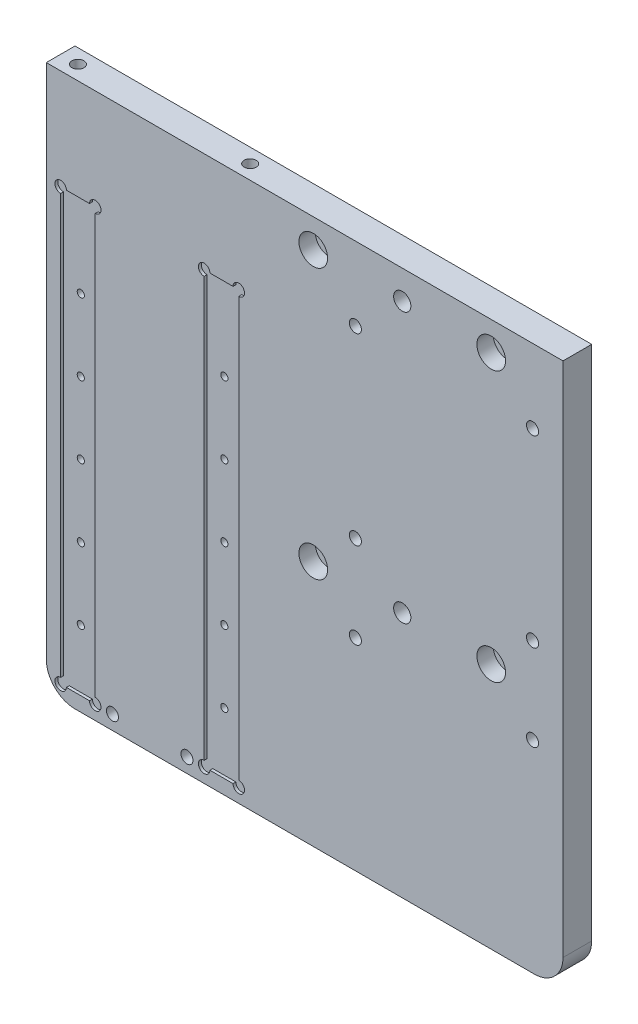
from build123d import *

# Parameters (mm, degrees)
SKETCH_1_W                = 180
SKETCH_1_H                = 190
EXTRUDE_1_DEPTH           = 10
HOLE_WIZARD_1_D           = 5.5
HOLE_WIZARD_1_CBORE_D     = 10
HOLE_WIZARD_1_CBORE_DEPTH = 5.7
PATTERN_LINEAR_1_COUNT    = 2
PATTERN_LINEAR_1_PITCH    = 94
SKETCH_4_W                = 12.05
SKETCH_4_H                = 150
CUT_EXTRUDE_1_DEPTH       = 1
SKETCH_6_R                = 2
CUT_EXTRUDE_2_DEPTH       = 1
HOLE_WIZARD_M5_1_D        = 4.2
HOLE_WIZARD_M5_1_DEPTH    = 14
HOLE_WIZARD_M5_1_TIP      = 1.2618073
FILLET_1_R                = 10
HOLE_WIZARD_M5_2_D        = 4.2
HOLE_WIZARD_M5_3_D        = 4.2
HOLE_WIZARD_6_0_6_1_D     = 6
HOLE_WIZARD_6_0_6_1_DEPTH = 10
HOLE_WIZARD_6_0_6_1_TIP   = 1.802581857
HOLE_WIZARD_M3_1_D        = 2.5


with BuildPart() as part:
    # 草图1 → 凸台-拉伸1 (new body)
    with BuildSketch(Plane.XY):
        with Locations((0, -95)):
            Rectangle(SKETCH_1_W, SKETCH_1_H)
    extrude(amount=EXTRUDE_1_DEPTH)

    # 打孔尺寸(%根据)开槽圆柱头螺钉的类型1 (through all)
    with Locations(Plane.XY.offset(10)):
        with Locations((65, -10), (3, -10)):
            hole_wizard_1 = CounterBoreHole(HOLE_WIZARD_1_D / 2, HOLE_WIZARD_1_CBORE_D / 2, HOLE_WIZARD_1_CBORE_DEPTH)

    # 阵列(线性)1: 打孔尺寸(%根据)开槽圆柱头螺钉的类型1 ×2
    with Locations(*[(0, -i * PATTERN_LINEAR_1_PITCH, 0) for i in range(1, PATTERN_LINEAR_1_COUNT)]):
        add(hole_wizard_1, mode=Mode.SUBTRACT)

    # 草图4 → 切除-拉伸1 (cut)
    with BuildSketch(Plane.XY.offset(10)):
        with Locations((-78.975, -110)):
            Rectangle(SKETCH_4_W, SKETCH_4_H)
        with Locations((-28.975, -110)):
            Rectangle(SKETCH_4_W, SKETCH_4_H)
    extrude(amount=-CUT_EXTRUDE_1_DEPTH, mode=Mode.SUBTRACT)

    # 草图6 → 切除-拉伸2 (cut)
    with BuildSketch(Plane.XY.offset(10)):
        with Locations((-72.95, -35)):
            Circle(SKETCH_6_R)
        with Locations((-85, -35)):
            Circle(SKETCH_6_R)
        with Locations((-85, -185)):
            Circle(SKETCH_6_R)
        with Locations((-72.95, -185)):
            Circle(SKETCH_6_R)
        with Locations((-35, -185)):
            Circle(SKETCH_6_R)
        with Locations((-22.95, -185)):
            Circle(SKETCH_6_R)
        with Locations((-35, -35)):
            Circle(SKETCH_6_R)
        with Locations((-22.95, -35)):
            Circle(SKETCH_6_R)
    extrude(amount=-CUT_EXTRUDE_2_DEPTH, mode=Mode.SUBTRACT)

    # M5 螺纹孔1
    with Locations(Plane(origin=(0, 0, 0), x_dir=(1, 0, 0), z_dir=(0, 1, 0))):
        with Locations((-23.975, -5), (-83.975, -5)):
            Hole(HOLE_WIZARD_M5_1_D / 2, depth=HOLE_WIZARD_M5_1_DEPTH)
            with Locations((0, 0, -(HOLE_WIZARD_M5_1_DEPTH + HOLE_WIZARD_M5_1_TIP / 2))):  # 118° drill point
                Cone(0, HOLE_WIZARD_M5_1_D / 2, HOLE_WIZARD_M5_1_TIP, mode=Mode.SUBTRACT)

    # 圆角1
    fillet_1_edges = [part.edges().sort_by_distance(p)[0] for p in [
        (90, -190, 5),
        (-90, -190, 5),
    ]]
    fillet(fillet_1_edges, radius=FILLET_1_R)

    # M5 螺纹孔2 (through all)
    with Locations(Plane.XY.offset(10)):
        with Locations((-66.95, -185), (-41, -185)):
            Hole(HOLE_WIZARD_M5_2_D / 2)

    # M5 螺纹孔3 (through all)
    with Locations(Plane.XY.offset(10)):
        with Locations((79.379496826, -119.666387024), (17.670502343, -119.666387024), (17.670502343, -89.666387024), (79.379496826, -89.666387024), (79.379496826, -25.666387024), (17.670502343, -25.666387024)):
            Hole(HOLE_WIZARD_M5_3_D / 2)

    # Ø6.0 (6) 直径孔1
    with Locations(Plane.XY.offset(10)):
        with Locations((34, -104), (34, -10)):
            Hole(HOLE_WIZARD_6_0_6_1_D / 2, depth=HOLE_WIZARD_6_0_6_1_DEPTH)
            with Locations((0, 0, -(HOLE_WIZARD_6_0_6_1_DEPTH + HOLE_WIZARD_6_0_6_1_TIP / 2))):  # 118° drill point
                Cone(0, HOLE_WIZARD_6_0_6_1_D / 2, HOLE_WIZARD_6_0_6_1_TIP, mode=Mode.SUBTRACT)

    # M3 螺纹孔1 (through all)
    with Locations(Plane.XY.offset(10)):
        with Locations((-28.975, -64.7), (-78.975, -64.7), (-78.975, -89.7), (-78.975, -114.7), (-78.975, -164.7), (-78.975, -139.7), (-28.975, -164.7), (-28.975, -139.7), (-28.975, -114.7), (-28.975, -89.7)):
            Hole(HOLE_WIZARD_M3_1_D / 2)


solid = part.part
